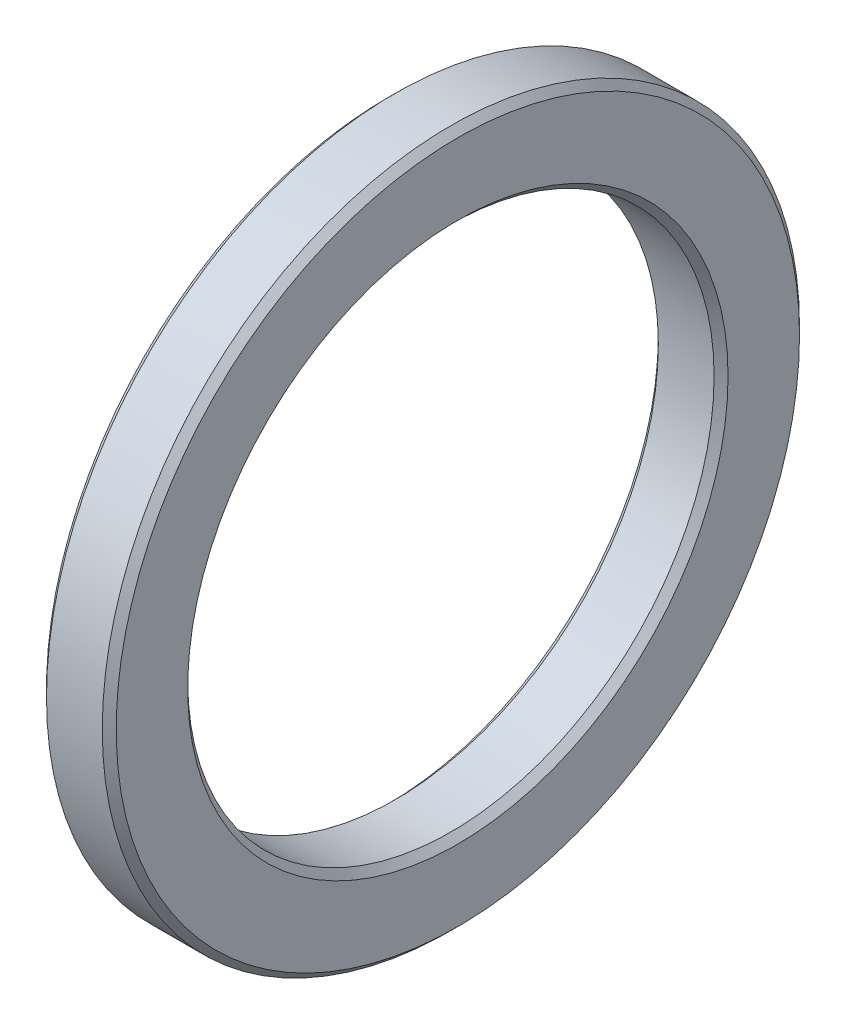
from build123d import *

# Parameters (mm, degrees)
SKETCH_1_R      = 10
SKETCH_1_R_2    = 7.55
EXTRUDE_1_DEPTH = 2
CHAMFER_1_SIZE  = 0.2


with BuildPart() as part:
    # 草图1 → 凸台-拉伸1 (new body)
    with BuildSketch(Plane(origin=(0, 0, 0), x_dir=(0, 0, -1), z_dir=(1, 0, 0))):
        Circle(SKETCH_1_R)
        Circle(SKETCH_1_R_2, mode=Mode.SUBTRACT)
    extrude(amount=EXTRUDE_1_DEPTH)

    # 倒角1
    chamfer_1_edges = [part.edges().sort_by_distance(p)[0] for p in [
        (0, 0, 10),
        (2, 0, 10),
        (0, 0, 7.55),
        (2, 0, 7.55),
    ]]
    chamfer(chamfer_1_edges, length=CHAMFER_1_SIZE)


solid = part.part
